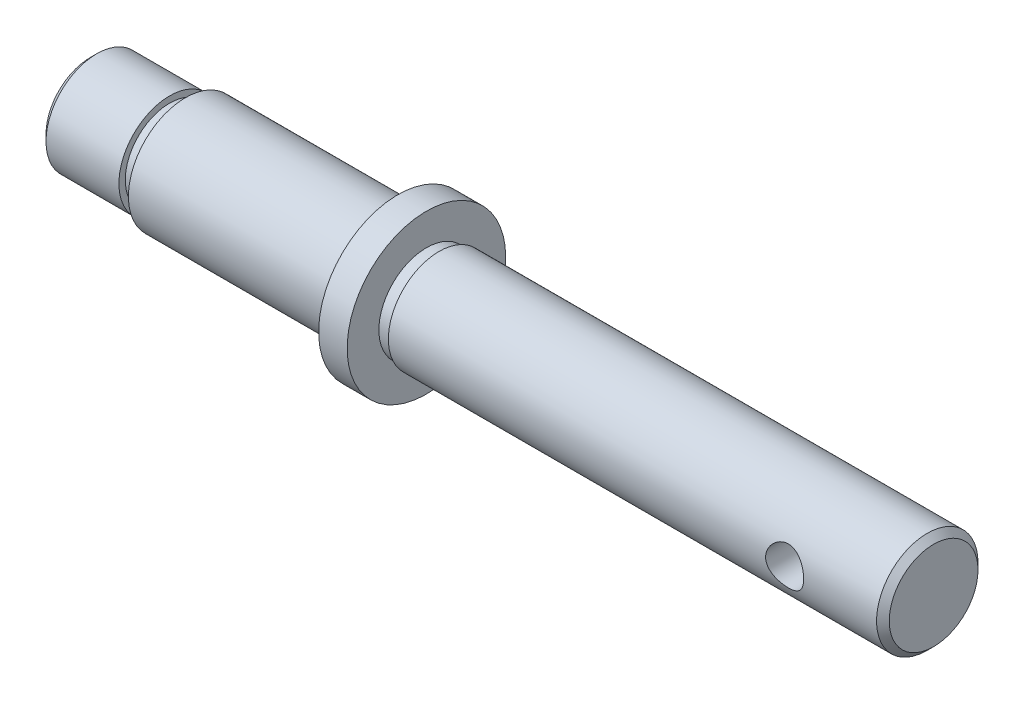
SolidWorks part; units mm, degrees
ref_plane "Front Plane" through (0, 0, 0) normal (0, 0, 1) x (1, 0, 0)
ref_plane "Top Plane" through (0, 0, 0) normal (0, 1, 0) x (1, 0, 0)
ref_plane "Right Plane" through (0, 0, 0) normal (1, 0, 0) x (0, 0, -1)
other "Configuration Table"
sketch "Sketch1" plane through (0, 0, 0) normal (0, 0, 1) x (1, 0, 0)
  line L0 (0, 0) -> (0, 8)
  line L1 (0, 8) -> (12.5, 8)
  line L2 (12.5, 8) -> (12.5, 7)
  line L3 (12.5, 7) -> (15, 7)
  line L4 (15, 7) -> (15, 9)
  line L5 (15, 9) -> (46.5, 9)
  line L6 (46.5, 9) -> (46.5, 8.5)
  line L7 (46.5, 8.5) -> (48.5, 8.5)
  line L8 (48.5, 8.5) -> (48.5, 12.5)
  line L9 (48.5, 12.5) -> (53, 12.5)
  line L10 (53, 12.5) -> (53, 7.5)
  line L11 (53, 7.5) -> (55, 7.5)
  line L12 (55, 7.5) -> (55, 8)
  line L13 (55, 8) -> (133, 8)
  line L14 (133, 8) -> (133, 0)
  line L15 (133, 0) -> (0, 0) construction
  line L16 (0, 0) -> (133, 0)
  point P14 (48.5, 10.5)
  dimension "D1" = 133
  dimension "D2" = 16
  dimension "D3" = 2.5
  dimension "D4" = 1
  dimension "D5" = 18
  dimension "D6" = 33.5
  dimension "D7" = 2
  dimension "D8" = 0.5
  dimension "D9" = 48.5
  dimension "D10" = 25
  dimension "D11" = 4.5
  dimension "D12" = 2
  dimension "D13" = 0.5
  dimension "D14" = 16
revolve "Revolve1" add sketch "Sketch1" angle 360 about L15
cosmetic thread "Cosmetic Thread1" parameters "D2"=13.835
sketch "Sketch2" plane through (0, 0, 0) normal (0, 0, 1) x (1, 0, 0)
  line L0 (53, -12.5) -> (53, 12.5) construction
  circle A0 centre (117.5, 0) radius 3
  dimension "D1" = 6
  dimension "D2" = 64.5
extrude "Cut-Extrude1" cut sketch "Sketch2" against normal through all both and the other way through all
sketch "Sketch3" plane through (0, 0, 0) normal (-1, 0, 0) x (0, 0, 1)
  circle A0 centre (0, 0) radius 3
  dimension "D1" = 6
extrude "Cut-Extrude2" cut sketch "Sketch3" against normal blind 8 and the other way through all
sketch "Sketch4" plane through (8, 0, 0) normal (-1, 0, 0) x (0, 0, 1)
  circle A0 centre (0, 0) radius 1.5
  dimension "D1" = 3
extrude "Cut-Extrude3" cut sketch "Sketch4" against normal blind 50
sketch "Sketch5" plane through (0, 0, 0) normal (0, 0, 1) x (1, 0, 0)
  line L0 (58, 1.5) -> (58, -1.5)
  arc A0 (58, -1.5) -> (58, 1.5) centre (58, 0) ccw
  dimension "D2" = 3
  dimension "D1" = 58
chamfer "Chamfer1" distance 1.5 angle 30 1 edges at (0, 0, 3)
chamfer "Chamfer2" distance 1 angle 45 2 edges at (133, 0, -8) (0, 0, -8)
revolve "Cut-Revolve1" cut sketch "Sketch5" angle 360 about L0
